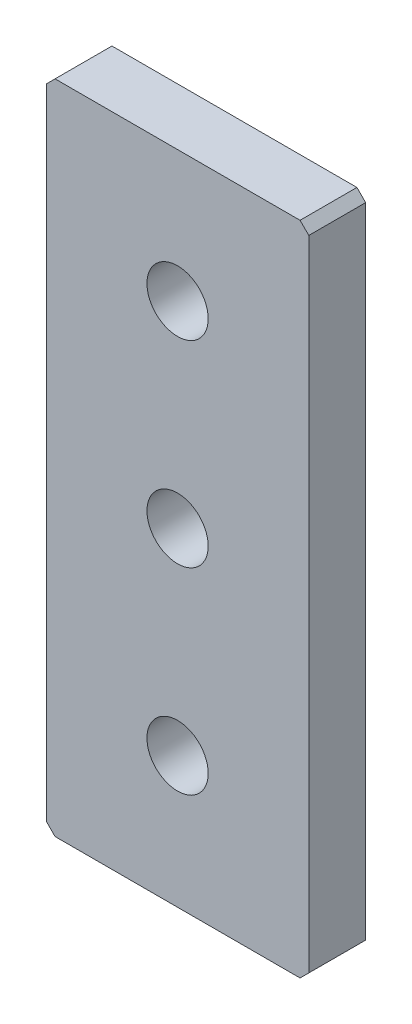
SolidWorks part; units mm, degrees
ref_plane "前视基准面" through (0, 0, 0) normal (0, 0, 1) x (1, 0, 0)
ref_plane "上视基准面" through (0, 0, 0) normal (0, 1, 0) x (1, 0, 0)
ref_plane "右视基准面" through (0, 0, 0) normal (1, 0, 0) x (0, 0, -1)
sketch "草图1" plane through (0, 0, 0) normal (0, 0, 1) x (1, 0, 0)
  line L1 (-15, 37.5) -> (15, 37.5)
  line L2 (-15, 37.5) -> (-15, -37.5)
  line L3 (-15, -37.5) -> (15, -37.5)
  line L4 (15, 37.5) -> (15, -37.5)
  line L5 (-15, 37.5) -> (15, -37.5) construction
  line L6 (-15, -37.5) -> (15, 37.5) construction
  point P0 (0, 0)
  dimension "D1" = 30
  dimension "D2" = 75
extrude "凸台-拉伸1" add sketch "草图1" along normal blind 6.5
hole_wizard "Ø7.0 (7) 直径孔1" positions "草图5" profile "草图4" hole size "Ø7.0" standard "ISO" end condition through all
sketch "草图5" plane through (0, 0, 6.5) normal (0, 0, 1) x (1, 0, 0)
  point P0 (0, 0)
  point P3 (0, -22.5)
  point P5 (0, 22.5)
  dimension "D1" = 45
  dimension "D2" = 22.5
sketch "草图4" plane through (0, 0, 6.5) normal (1, 0, 0) x (0, -1, 0)
  line L0 (0, 0) -> (0, 6.5)
  line L1 (0, 6.5) -> (3.5, 6.5)
  line L2 (3.5, 6.5) -> (3.5, 0)
  line L5 (3.5, 0) -> (0, 0)
  line L11 (0, -6.35) -> (0, 107.95) construction
  dimension "通孔孔直径" = 7
  dimension "通孔孔深度" = 6.5
chamfer "倒角1" distance 1 angle 45 4 edges at (-15, 37.5, 3.25) (15, 37.5, 3.25) (15, -37.5, 3.25) (-15, -37.5, 3.25)
